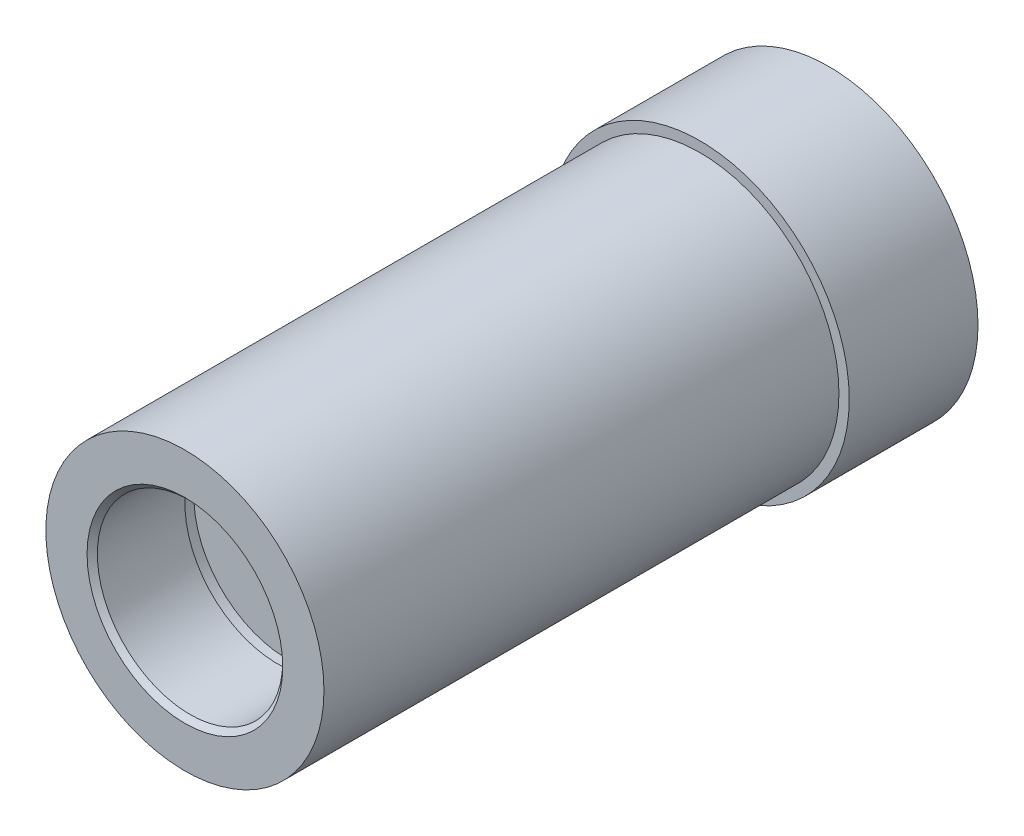
from build123d import *

# Parameters (mm, degrees)
SKETCH1_R           = 29
BOSS_EXTRUDE1_DEPTH = 25
SKETCH2_R           = 27
BOSS_EXTRUDE2_DEPTH = 100
SKETCH7_R           = 24
CUT_EXTRUDE4_DEPTH  = 22
SKETCH8_R           = 24.1
CUT_EXTRUDE5_DEPTH  = 3
CHAMFER1_SIZE       = 1
SKETCH9_R           = 18
CUT_EXTRUDE6_DEPTH  = 18
SKETCH10_R          = 18.25
CUT_EXTRUDE7_DEPTH  = 2
CHAMFER2_SIZE       = 1


with BuildPart() as part:
    # Sketch1 → Boss-Extrude1 (new body)
    with BuildSketch(Plane.XY):
        Circle(SKETCH1_R)
    extrude(amount=BOSS_EXTRUDE1_DEPTH)

    # Sketch2 → Boss-Extrude2 (add)
    with BuildSketch(Plane.XY.offset(25)):
        Circle(SKETCH2_R)
    extrude(amount=BOSS_EXTRUDE2_DEPTH)

    # Sketch7 → Cut-Extrude4 (cut)
    with BuildSketch(Plane(origin=(0, 0, 0), x_dir=(-1, 0, 0), z_dir=(0, 0, -1))):
        Circle(SKETCH7_R)
    extrude(amount=-CUT_EXTRUDE4_DEPTH, mode=Mode.SUBTRACT)

    # Sketch8 → Cut-Extrude5 (cut)
    with BuildSketch(Plane(origin=(0, 0, 22), x_dir=(-1, 0, 0), z_dir=(0, 0, -1))):
        Circle(SKETCH8_R)
    extrude(amount=-CUT_EXTRUDE5_DEPTH, mode=Mode.SUBTRACT)

    # Chamfer1
    chamfer1_edges = [part.edges().sort_by_distance(p)[0] for p in [
        (24, 0, 0),
    ]]
    chamfer(chamfer1_edges, length=CHAMFER1_SIZE)

    # Sketch9 → Cut-Extrude6 (cut)
    with BuildSketch(Plane.XY.offset(125)):
        Circle(SKETCH9_R)
    extrude(amount=-CUT_EXTRUDE6_DEPTH, mode=Mode.SUBTRACT)

    # Sketch10 → Cut-Extrude7 (cut)
    with BuildSketch(Plane.XY.offset(107)):
        Circle(SKETCH10_R)
    extrude(amount=-CUT_EXTRUDE7_DEPTH, mode=Mode.SUBTRACT)

    # Chamfer2
    chamfer2_edges = [part.edges().sort_by_distance(p)[0] for p in [
        (-18, 0, 125),
    ]]
    chamfer(chamfer2_edges, length=CHAMFER2_SIZE)


solid = part.part
